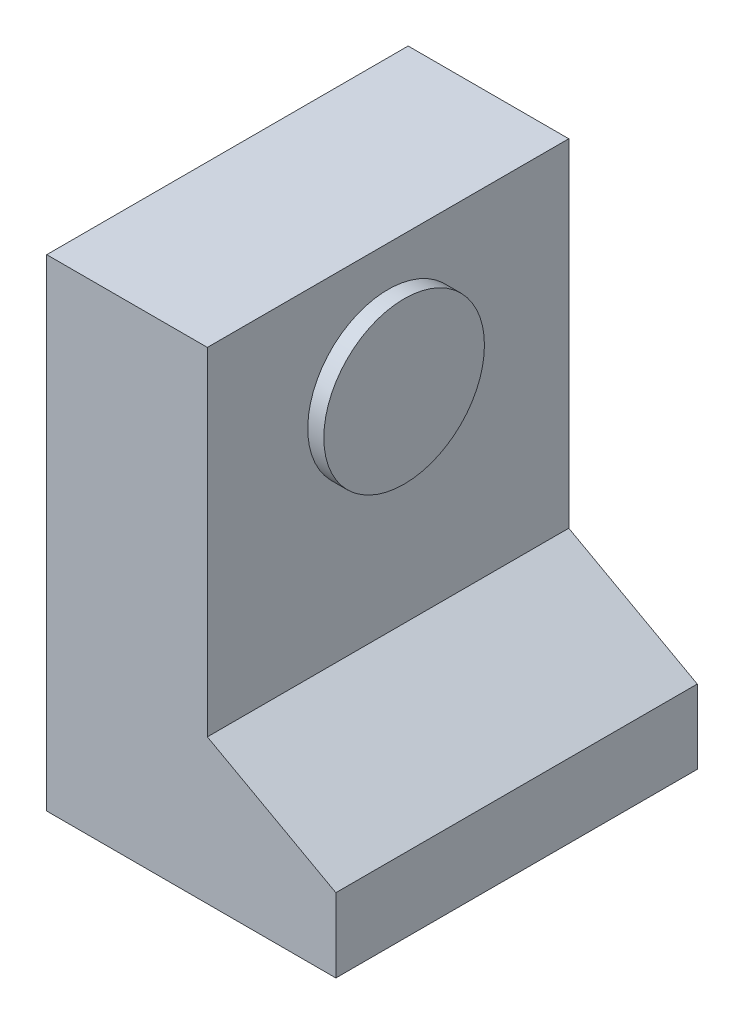
from build123d import *

# Parameters (mm, degrees)
SKETCH1_W           = 450
SKETCH1_H           = 600
BOSS_EXTRUDE1_DEPTH = 400
CUT_EXTRUDE1_DEPTH  = 2400
SKETCH4_W           = 648.804514889
SKETCH4_H           = 183.272574448
CUT_EXTRUDE2_DEPTH  = 40
SKETCH5_R           = 100
BOSS_EXTRUDE2_DEPTH = 20


with BuildPart() as part:
    # Sketch1 → Boss-Extrude1 (new body)
    with BuildSketch(Plane(origin=(0, 0, 0), x_dir=(0, 0, -1), z_dir=(1, 0, 0))):
        Rectangle(SKETCH1_W, SKETCH1_H)
    extrude(amount=BOSS_EXTRUDE1_DEPTH)

    # Sketch2 → Cut-Extrude1 (cut)
    with BuildSketch(Plane.XY.offset(225)):
        Polygon((200, 300), (200, -120), (400, -230), (400, 300), align=None)
    extrude(amount=-CUT_EXTRUDE1_DEPTH, mode=Mode.SUBTRACT)

    # Sketch4 → Cut-Extrude2 (cut)
    with BuildSketch(Plane(origin=(400, 0, 0), x_dir=(0, 0, -1), z_dir=(1, 0, 0))):
        with Locations((-2.450168107, -263.148054755)):
            Rectangle(SKETCH4_W, SKETCH4_H)
    extrude(amount=-CUT_EXTRUDE2_DEPTH, mode=Mode.SUBTRACT)

    # Sketch5 → Boss-Extrude2 (add)
    with BuildSketch(Plane(origin=(200, 0, 0), x_dir=(0, 0, -1), z_dir=(1, 0, 0))):
        with Locations(Location((0, 150, 0), (0, 0, 270))):
            Circle(SKETCH5_R)
    extrude(amount=BOSS_EXTRUDE2_DEPTH)


solid = part.part
